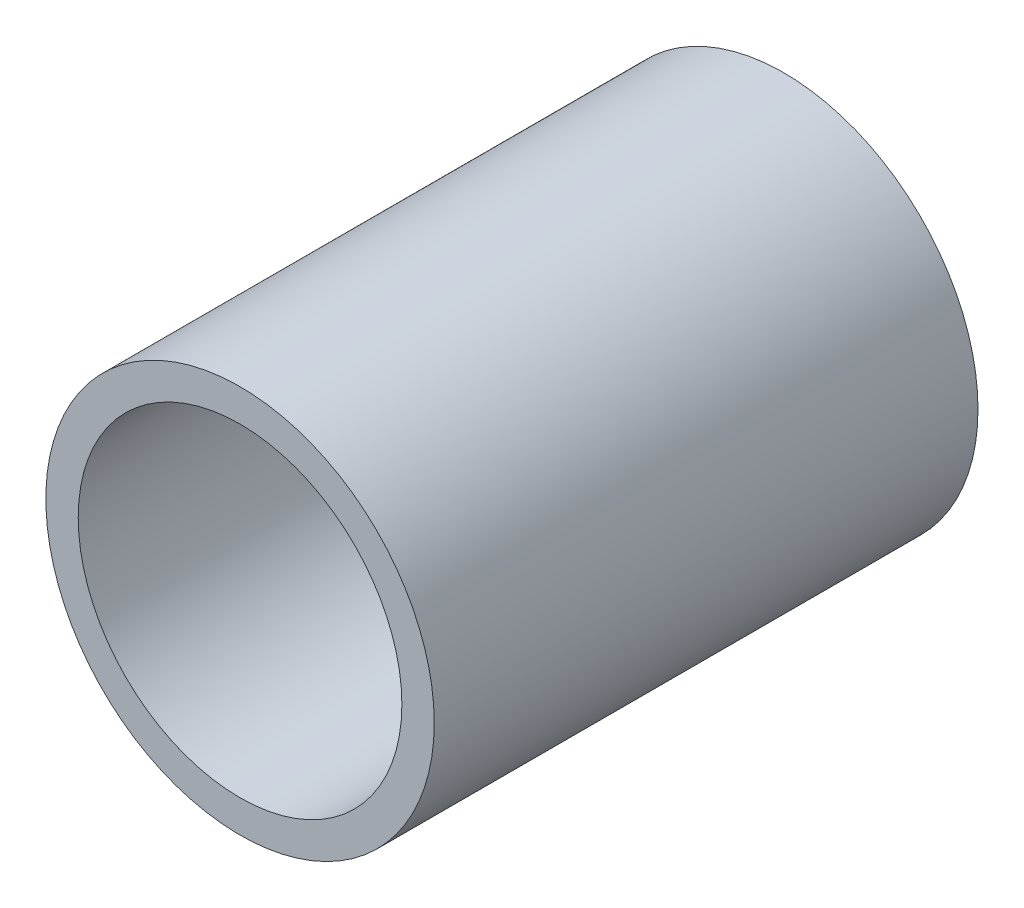
from build123d import *

# Parameters (mm, degrees)
SKETCH1_R           = 6
SKETCH1_R_2         = 5
BOSS_EXTRUDE1_DEPTH = 8.4


with BuildPart() as part:
    # Sketch1 → Boss-Extrude1 (new, symmetric)
    with BuildSketch(Plane.XY):
        Circle(SKETCH1_R)
        Circle(SKETCH1_R_2, mode=Mode.SUBTRACT)
    extrude(amount=BOSS_EXTRUDE1_DEPTH, both=True)


solid = part.part
